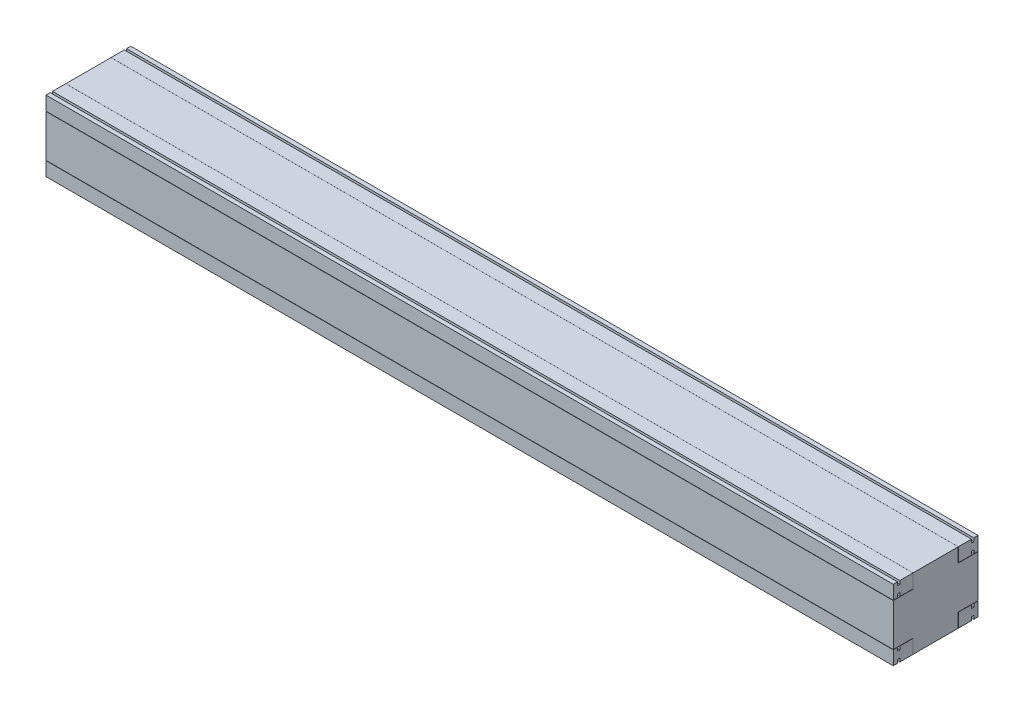
from build123d import *

# Parameters (mm, degrees)
SKETCH1_W           = 3000
SKETCH1_H           = 300
BOSS_EXTRUDE1_DEPTH = 250
SKETCH2_W           = 70
SKETCH2_H           = 50
CUT_EXTRUDE1_DEPTH  = 3015.13337462
BOSS_EXTRUDE2_DEPTH = 3000


with BuildPart() as part:
    # Sketch1 → Boss-Extrude1 (new body)
    with BuildSketch(Plane(origin=(0, 0, 0), x_dir=(1, 0, 0), z_dir=(0, 1, 0))):
        Rectangle(SKETCH1_W, SKETCH1_H)
    extrude(amount=BOSS_EXTRUDE1_DEPTH)

    # Sketch2 → Cut-Extrude1 (cut, through all)
    with BuildSketch(Plane(origin=(1500, 0, 0), x_dir=(0, 0, -1), z_dir=(1, 0, 0))):
        with Locations((-115, 225)):
            Rectangle(SKETCH2_W, SKETCH2_H)
        with Locations((-115, 25)):
            Rectangle(SKETCH2_W, SKETCH2_H)
        with Locations((115, 225)):
            Rectangle(SKETCH2_W, SKETCH2_H)
        with Locations((115, 25)):
            Rectangle(SKETCH2_W, SKETCH2_H)
    extrude(amount=-CUT_EXTRUDE1_DEPTH, mode=Mode.SUBTRACT)


with BuildPart() as body_2:
    # Sketch3 → Boss-Extrude2 (new body)
    with BuildSketch(Plane(origin=(1500, 0, 0), x_dir=(0, 0, -1), z_dir=(1, 0, 0))):
        Polygon((135, 250), (135, 238), (127, 238), (127, 250), (80.2, 250), (80.2, 201), (127, 201), (127, 213), (135, 213), (135, 201), (150, 201), (150, 250), align=None)
    extrude(amount=-BOSS_EXTRUDE2_DEPTH)


with BuildPart() as body_3:
    # Mirror3: mirrored copy
    add(body_2.part.mirror(Plane(origin=(0, 125, 0), x_dir=(0, 0, 1), z_dir=(0, -1, 0))))


with BuildPart() as body_4:
    # Mirror4: mirrored copy
    add(body_3.part.mirror(Plane.XY))


with BuildPart() as body_5:
    # Mirror4 2: mirrored copy
    add(body_2.part.mirror(Plane.XY))


solid = Compound([part.part, body_2.part, body_3.part, body_4.part, body_5.part])
